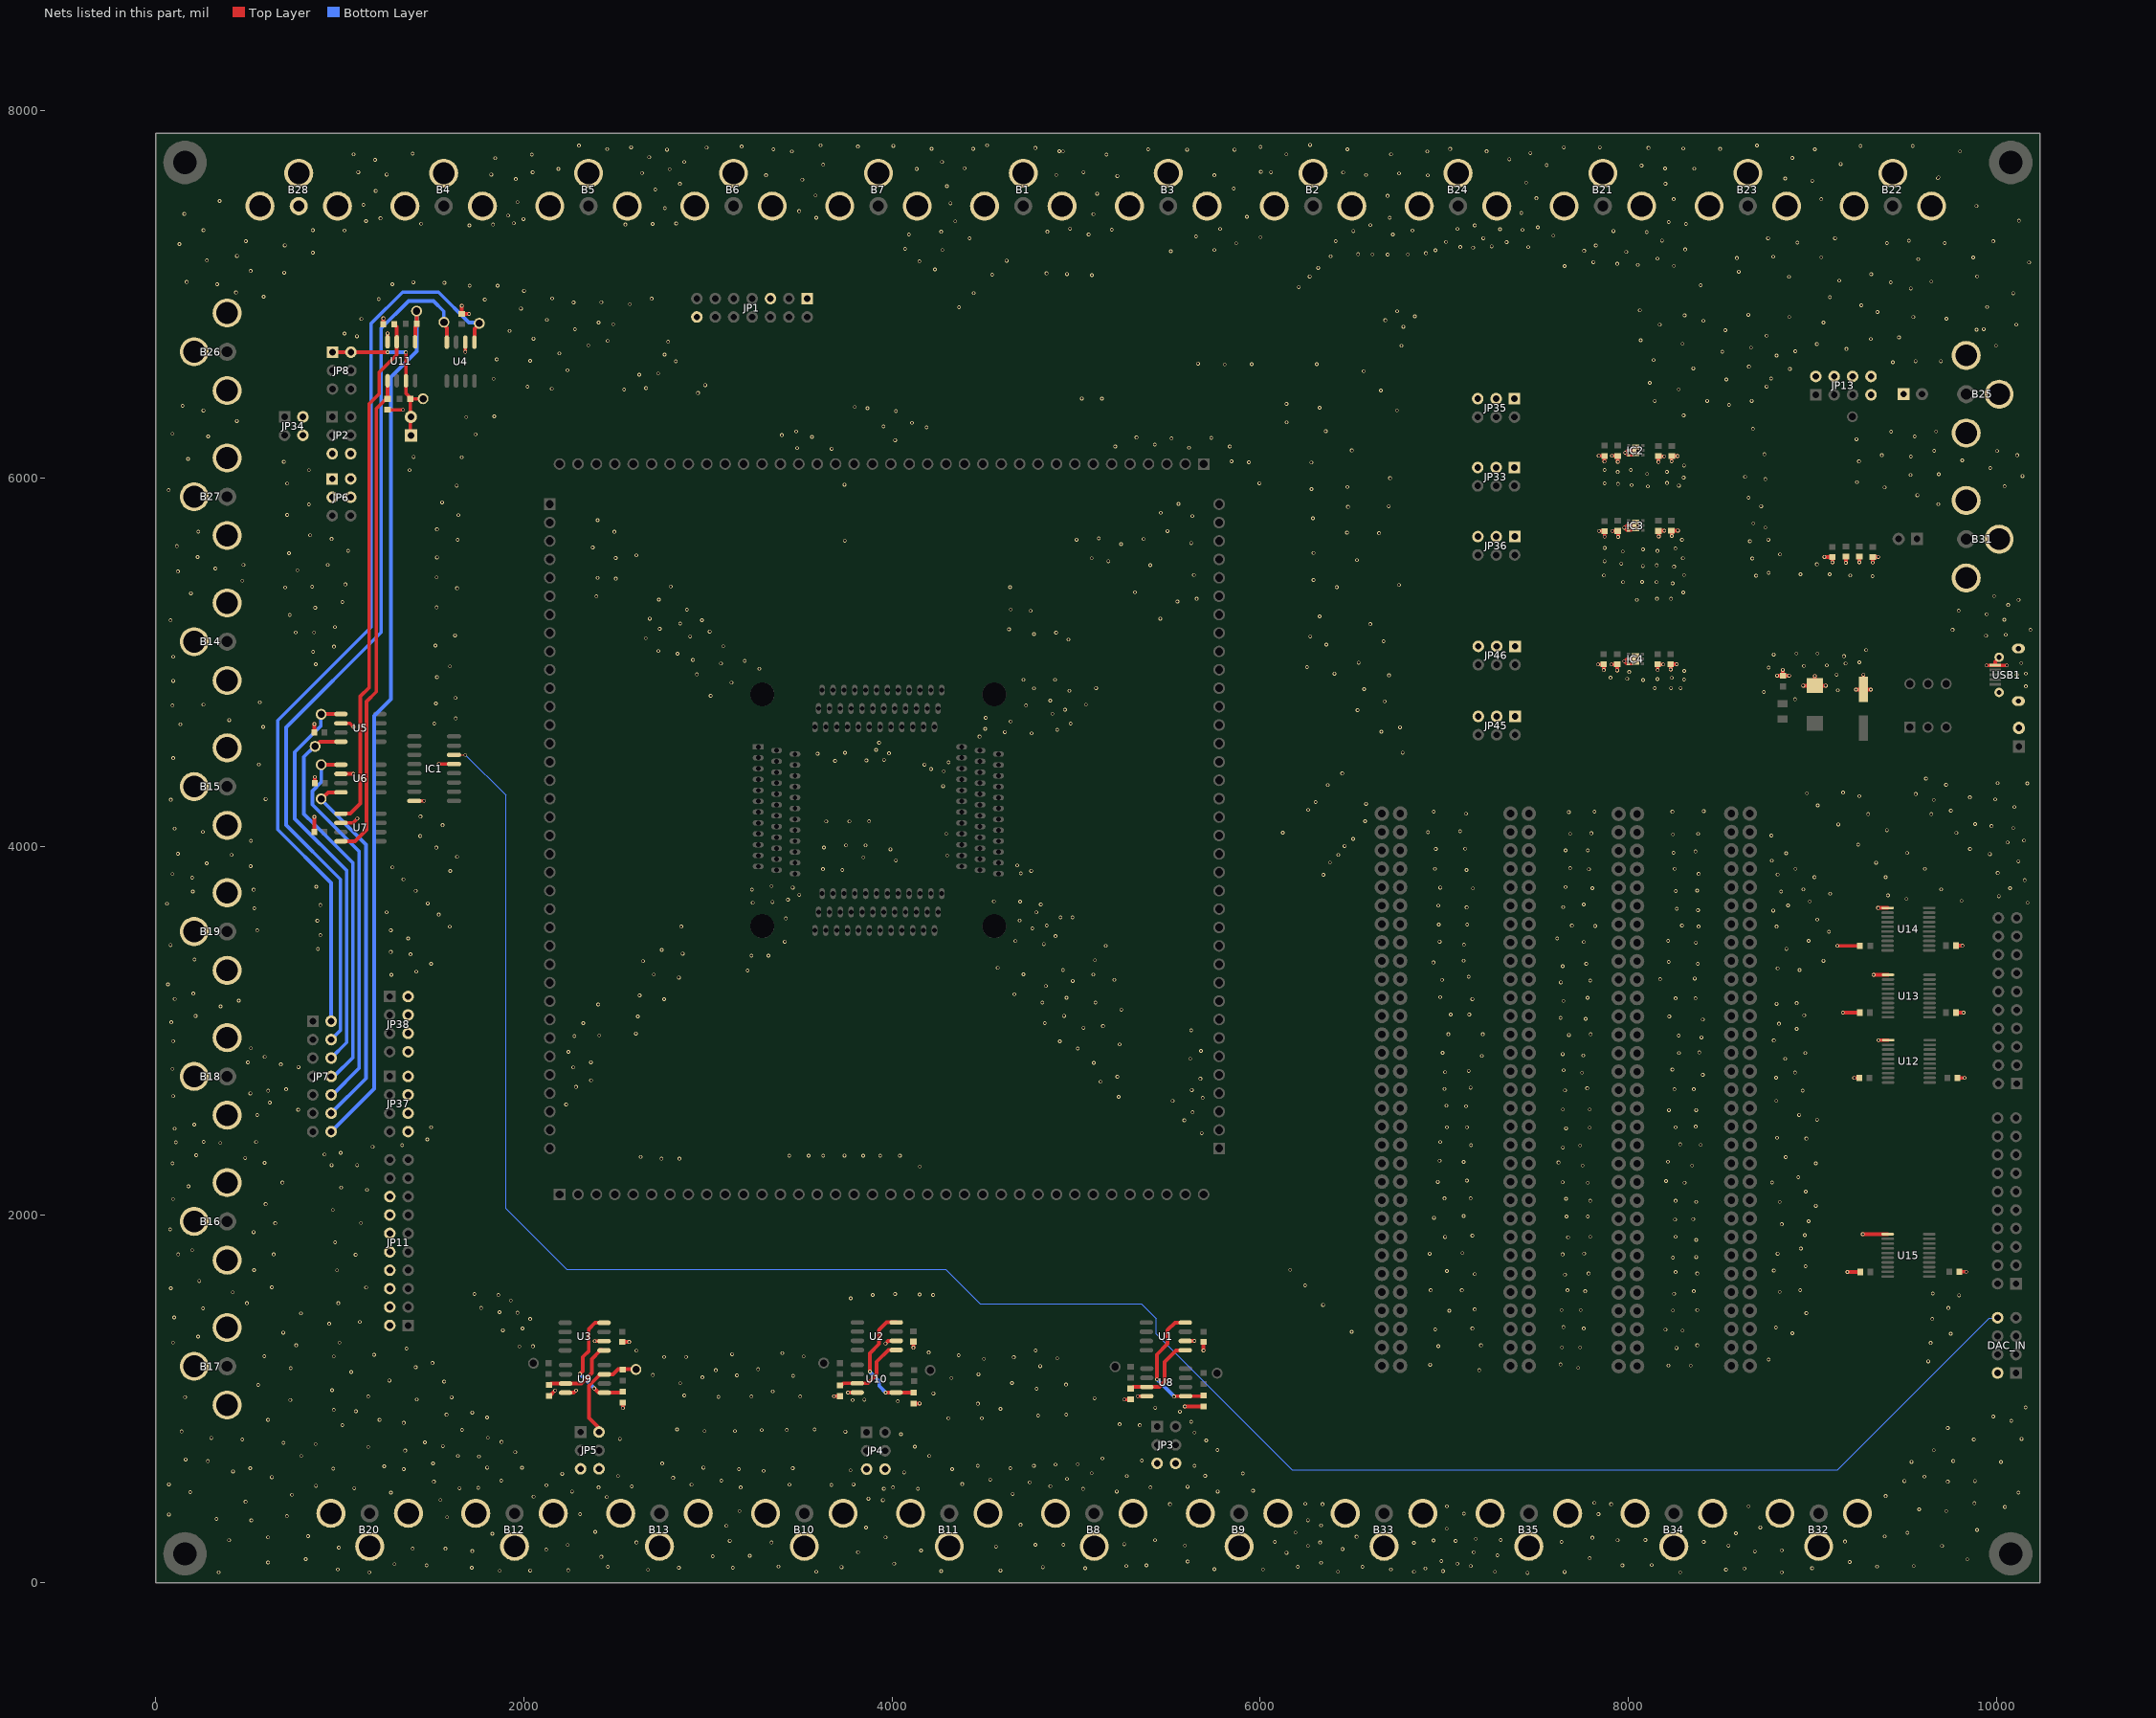
[diagram p0: the nets of this part, all layers, seen from the top]
# Altium PCB MISC62794.PcbDoc (part 3 of 7)
Units mil, origin at the board's own origin, x right, y up, seen from the top; angles counter-clockwise.
Board outline 10236.22 x 7874.02 mil, 4 copper layers (Top Layer, GND, POWER, Bottom Layer); 158 components, 185 nets, 1211 pads, 1759 vias.

## Via types
v1: diameter 20, hole 12, Top Layer to Bottom Layer, 1759 vias

## Nets (pads, with @x,y where several pads share a name; then routed paths per layer and width w, separated by ;. In a path a pad name is that pad's centre, name@x,y a point inside that pad or via, vN(x,y) a via of type N, cw(c..) or ccw(c..) an arc to the next point about the centre after c; other vN are vias at no path point) (continued)
DAC6: JP5.2 R11.1 TP6.1 U9.7 | length 549.3
  Top Layer w20: JP5.2@2407.19,819.02 2407.19,840.81 2353,895 2353,1071 2414,1132 U9.7@2429,1132 ; U9.7@2436.73,1132.67 2483.67,1132.67 2511,1160 TP6.1@2599,1160
DAC7: JP7.2 TP7.1 U4.5 | length 4943.5
  Top Layer w20: U4.5@1730.71,6740.23 1730.71,6812.71 TP7.1@1751,6833
  Bottom Layer w20: JP7.2@952,3051 952,3802 662,4092 662,4685 1169,5192 1169,6841 1340,7012 1535,7012 1700,6847 TP7.1@1752,6847
DAC8: JP7.4 TP8.1 U4.8 | length 4799.4
  Top Layer w20: TP8.1@1566,6833 1580.71,6818.29 U4.8@1580.71,6740.23
  Bottom Layer w20: JP7.4@952,2951 1002,3001 1002,3822 707,4117 707,4647 1223,5163 1223,6177 ; 1223,6188 1223,6177 ; TP8.1@1564,6865 1564,6908 1508,6964 1372,6964 1223,6815 1223,6177
DAC9: JP7.6 TP9.1 U5.5 | length 2171.8
  Top Layer w20: TP9.1@906.54,4719.46 U5.5@1004.93,4719.46
  Bottom Layer w20: TP9.1@896,4714 896,4655 754,4513 754,4151 1036,3869 1036,2935 JP7.6@952,2851
DAC10: JP7.8 TP10.1 U5.8 | length 2132.1
  Top Layer w20: TP10.1@866,4545 890.46,4569.46 U5.8@1004.93,4569.46
  Bottom Layer w20: TP10.1@860,4543 804,4487 804,4177 860,4121 1070,3911 1070,2854 967,2751 JP7.8@952,2751
DAC11: JP7.10 TP11.1 U6.5 | length 2057.5
  Top Layer w20: TP11.1@917.54,4444.46 U6.5@1004.93,4444.46
  Bottom Layer w20: TP11.1@898,4429 898,4350 850,4302 850,4227 1104,3973 1104,2796 959,2651 JP7.10@952,2651
DAC12: JP7.12 TP12.1 U6.8 | length 1981.8
  Top Layer w20: TP12.1@908,4267 935.46,4294.46 U6.8@1004.93,4294.46
  Bottom Layer w20: TP12.1@904,4248 1141,4011 1141,2740 JP7.12@952,2551
DAC13: JP7.14 R13.2 TP13.1 U11.1 | length 4828.2
  Top Layer w20: U11.1@1408.29,6741.99 1408.29,6820.29 1417,6829 TP13.1@1417,6914
  Bottom Layer w20: JP7.14@952,2451 1185,2684 1185,4710 1276,4801 1276,6550 1417,6691 TP13.1@1417,6911
DAC14: JP8.1 JP8.2 JP20.1 JP20.2 R15.1 TP14.1 U11.7 | length 923.6
  Top Layer w20: JP8.1@959,6686.02 1006,6686.02 JP8.2@1059,6686.02 ; JP8.2@1066.98,6686.02 JP8.2@1059,6686.02 ; v1(1257.98,6686.02) JP8.2@1059,6686.02 ; v1@1358.29,6683.29 U11.7@1358.29,6530.77 1358.29,6461.71 R15.1@1386,6434 ; JP20.1@1381.95,6241.95 R15.1@1381.95,6432.38 TP14.1@1448.38,6432.38
  Bottom Layer w20: v1(1257.98,6686.02) v1@1357,6686.02
  other v1: 1358,6685
DAC_OUT1: R2.1 U1.5 U8.3 | length 432.4
  Top Layer w20: R2.1@5303,1055 5311.67,1063.67 U8.3@5383.51,1063.67 5451.67,1063.67 5481,1093 5481,1200 5543,1262 U1.5@5587,1262
DAC_OUT2: R4.1 U1.8 U8.5 | length 691.7
  Top Layer w20: v1(5439,1105) 5439,1240 5497,1298 5497,1373 5537.67,1413.67 U1.8@5592.73,1413.67 ; v1(5532,1012) v1@5533,1012 ; v1@5533,1013 5533.67,1013.67 U8.5@5594.73,1013.67 R4.1@5687.33,1013.67
  Bottom Layer w20: v1(5439,1105) v1(5532,1012)
DAC_OUT3: R6.1 U2.5 U10.3 | length 399.7
  Top Layer w20: R6.1@3729,1078 3734.67,1083.67 U10.3@3810.51,1083.67 U10.3@3823,1083.67 ; U10.3@3823,1084 3868,1084 3916,1132 3916,1201 3980,1265 U2.5@4011,1265
DAC_OUT4: R8.1 U2.8 U10.5 | length 655.7
  Top Layer w20: v1(3879,1148) 3879,1247 3929,1297 3929,1373 3970.67,1414.67 U2.8@4022.73,1414.67 ; v1(3965.33,1033.67) U10.5@4021.73,1033.67 R8.1@4116.67,1033.67
  Bottom Layer w20: v1@3880,1146 3930,1096 3930,1069 v1(3965.33,1033.67)
DAC_OUT5: R10.1 U3.5 U9.3 | length 403.6
  Top Layer w20: R10.1@2140,1075 2147.67,1082.67 U9.3@2225.51,1082.67 2310.67,1082.67 2368,1140 2368,1216 U3.5@2413,1261 ; U3.5@2413,1264 U3.5@2422,1264
DAC_OUT6: R12.1 U3.8 U9.5 | length 633.7
  Top Layer w20: v1@2302,1134 v1@2302.5,1134.5 ; v1(2303,1134) v1@2302.5,1134.5 ; v1(2381,1056) 2404.33,1032.67 U9.5@2436.73,1032.67 R12.1@2531.67,1032.67 ; U3.8@2434.73,1412.67 2385.67,1412.67 2352,1379 2352,1260 2319,1227 2319,1151 v1@2302.5,1134.5
  Bottom Layer w20: v1(2303,1134) v1(2381,1056)
DAC_OUT13: R14.1 U7.5 U11.3 | length 2816.8
  Top Layer w20: U7.5@1004.93,4178.46 1055.46,4178.46 1111,4234 1111,4816 1158,4863 1158,6404 1213,6459 1213,6577 1307,6671 1307,6825 R14.1@1296,6836
DAC_OUT14: R16.1 U7.8 U11.5 | length 2649.2
  Top Layer w20: U7.8@1004.93,4028.46 1082.46,4028.46 1144,4090 1144,4788 1197,4841 1197,6378 1259,6440 U11.5@1259,6527
DCDC_OUT: JP13.7 JP30.1
DIO: DAC_IN.8 IC1.14 | length 11690.6
  Top Layer w6: IC1.14@1619.33,4498.08 v1(1681.08,4498.08)
  Bottom Layer w6: v1(1681.08,4498.08) 1901,4278.16 1901,2033 2232,1702 4292,1702 4478.5,1515.5 5353.5,1515.5 5434,1435 5434,1353 6173,614 9138,614 9961,1437 DAC_IN.8@9997,1437
GND: B1.2 B1.3 B1.4 B2.2 B2.3 B2.4 B3.2 B3.3 B3.4 B4.2 B4.3 B4.4 B5.2 B5.3 B5.4 B6.2 B6.3 B6.4 B7.2 B7.3 B7.4 B8.2 B8.3 B8.4 B9.2 B9.3 B9.4 B10.2 B10.3 B10.4 B11.2 B11.3 B11.4 B12.2 B12.3 B12.4 B13.2 B13.3 B13.4 B14.2 B14.3 B14.4 B15.2 B15.3 B15.4 B16.2 B16.3 B16.4 B17.2 B17.3 B17.4 B18.2 B18.3 B18.4 B19.2 B19.3 B19.4 B20.2 B20.3 B20.4 B21.2 B21.3 B21.4 B22.2 B22.3 B22.4 B23.2 B23.3 B23.4 B24.2 B24.3 B24.4 B25.2 B25.3 B25.4 B26.2 B26.3 B26.4 B27.2 B27.3 B27.4 B28.1 B28.2 B28.3 B28.4 B31.2 B31.3 B31.4 B32.2 B32.3 B32.4 B33.2 B33.3 B33.4 B34.2 B34.3 B34.4 B35.2 B35.3 B35.4 C1.1 C2.1 C3.1 C4.1 C5.1 C6.1 C7.1 C8.2 C9.2 C10.2 C11.2 C20.2 C21.2 C22.2 C23.2 C24.2 C25.2 C26.2 C27.2 C28.2 C30.1 C31.2 C32.1 C33.2 C34.1 C35.2 C36.1 C37.2 C38.2 C39.2 C40.2 C41.2 D1.2 DAC_IN.2 IC1.8 IC1.13 IC2.2 IC2.3 IC2.7 IC3.2 IC3.3 IC3.7 IC4.2 IC4.3 IC4.7 JP1.1 JP1.5 JP1.14 JP2.5 JP2.6 JP3.5 JP3.6 JP4.5 JP4.6 JP5.5 JP5.6 JP6.1 JP6.2 JP6.3 JP6.4 JP11.2 JP11.4 JP11.6 JP11.8 JP11.10 JP11.12 JP11.14 JP11.16 JP13.2 JP13.4 JP13.6 JP13.8 JP32.2 JP33.1 JP33.3 JP33.5 JP34.2 JP34.4 JP35.1 JP35.3 JP35.5 JP36.1 JP36.3 JP36.5 JP37.2 JP37.4 JP37.6 JP37.8 JP38.2 JP38.4 JP38.6 JP38.8 JP45.1 JP45.3 JP45.5 JP46.1 JP46.3 JP46.5 R2.2 R4.2 R6.2 R8.2 R10.2 R12.2 R14.2 R16.2 R20.2 U1.6 U2.6 U3.6 U4.6 U5.6 U6.6 U7.6 U8.4 U9.4 U10.4 U11.4 U12.11 U13.11 U14.11 U15.11 USB1.5 USB1.6 USB1.7 USB1.8 USB1.9 | length 4162.4
  Top Layer w16: v1@7978,5006 7990.58,4993.42 IC4.3@8000.61,4993.42 IC4.7@8019.58,4993.42 ; v1(7978,5007) 7990.02,5019.02 IC4.2@8000.61,5019.02 IC4.7@8021.98,5019.02 ; v1@7978,5731 7990.58,5718.42 IC3.3@8000.61,5718.42 ; v1(7978,5732) 7990.02,5744.02 IC3.2@8000.61,5744.02 ; v1@7983,6139 7995.58,6126.42 IC2.3@8005.61,6126.42 ; v1(7983,6140) 7995.02,6152.02 IC2.2@8005.61,6152.02 ; IC3.3@8001.61,5718.42 8018.42,5718.42 IC3.7@8022,5722 ; IC3.2@8001.61,5744.02 IC3.7@8023.98,5744.02 ; IC2.3@8002.61,6126.42 IC2.7@8023.42,6126.42 ; IC2.2@8002.61,6152.02 IC2.7@8023.02,6152.02
  Top Layer w20: C7.1@860.98,4079.46 v1(860.98,4160.98) ; C5.1@860.98,4619.46 v1(860.98,4664.98) ; C6.1@862.98,4344.46 v1(862.98,4377.98) ; U7.6@1004.93,4128.46 1070.46,4128.46 v1(1094,4152) ; U6.6@1004.93,4394.46 v1(1072.54,4394.46) ; U5.6@1004.93,4669.46 1054.54,4669.46 v1(1074,4650) ; R14.2@1235.63,6838.38 v1(1235.63,6869.63) ; R16.2@1258.29,6372.72 1259.01,6372 v1(1343,6372) ; U11.4@1258.29,6741.99 v1(1258.29,6787.71) ; IC1.8@1403.94,4248.08 v1(1456.92,4248.08) ; v1(1537.08,4448.08) IC1.13@1619.33,4448.08 ; v1(1662,6938) C4.1@1662,6893.56 v1(1701.44,6893.56) ; v1(1680.71,6687.29) U4.6@1680.71,6740.23 ; R10.2@2135.12,1015.01 2139.01,1015.01 v1(2169,1045) ; U9.4@2225.51,1032.67 2270.67,1032.67 v1(2283,1045) ; v1(2384.33,1312.67) U3.6@2434.73,1312.67 ; C3.1@2534.12,1308.11 v1(2570.89,1308.11) ; v1(2537,949) R12.2@2537,978.34 ; v1(3684.01,1014.01) R6.2@3717.12,1014.01 ; v1(3760.33,1033.67) U10.4@3810.51,1033.67 ; v1(3964,1300) 3978.67,1314.67 U2.6@4022.73,1314.67 ; v1(4116.12,1277.12) C2.1@4116.12,1310.11 ; R8.2@4118,974.34 v1(4149.34,974.34) ; v1(5260.99,996.01) R2.2@5296.12,996.01 ; v1(5334,1014) 5334.33,1013.67 U8.4@5383.51,1013.67 ; v1(5590.66,958.34) R4.2@5693,958.34 ; U1.6@5592.73,1313.67 v1(5643.33,1313.67) ; v1(5692.12,1262.12) C1.1@5692.12,1309.11 ; v1(7835.54,4989.46) C41.2@7866.56,4989.46 v1(7866.56,4958.44) ; v1(7839.54,6122.46) 7870.56,6122.46 v1(7870.56,6091.44) ; v1(7840.54,5714.46) 7871.56,5714.46 v1(7871.56,5683.44) ; v1(7907.54,4989.46) C40.2@7939.56,4989.46 v1(7939.56,4957.44) ; v1(7911.54,6122.46) 7943.56,6122.46 v1(7943.56,6090.44) ; v1(7912.54,5714.46) 7944.56,5714.46 v1(7944.56,5682.44) ; v1(8159.56,4958.44) C38.2@8159.56,4989.46 v1(8190.54,4989.46) ; v1(8164.56,6089.44) C24.2@8164.56,6120.46 v1(8195.54,6120.46) ; v1(8165.56,5684.44) 8165.56,5715.46 v1(8196.54,5715.46) ; v1(8230.56,4961.56) C39.2@8230.56,4990.46 v1(8263.54,4990.46) ; v1(8235.56,6092.56) 8235.56,6121.46 v1(8268.54,6121.46) ; v1(8236.56,5687.56) 8236.56,5716.46 v1(8269.54,5716.46) ; v1(8808.34,4928.66) R20.2@8840,4928.66 ; v1(8840,4960) R20.2@8840,4928.66 ; v1(8874.34,4928.66) R20.2@8840,4928.66 ; v1(8950.98,4874.02) D1.2@9014,4874.02 ; v1(9014,4927) D1.2@9014,4874.02 ; v1(9065.59,5573.41) C10.2@9109.29,5573.41 v1(9109.29,5544.29) ; v1(9072.98,4874.02) D1.2@9014,4874.02 ; v1(9135.99,3460.01) C34.1@9259.44,3460.01 ; v1(9165.99,3098.01) C32.1@9257.44,3098.01 ; v1(9182.29,5541.29) C9.2@9182.29,5574.41 ; v1(9191.01,1689.01) C36.1@9260.44,1689.01 ; v1(9228,2743) C30.1@9255.44,2743.01 ; v1(9237.12,4853.12) C20.2@9278,4853.12 ; v1(9255.29,5544.29) C8.2@9255.29,5575.41 ; v1(9274.83,1894.17) U15.11@9409.97,1894.17 ; v1(9278,4934) C20.2@9278,4853.12 ; v1(9317.88,4853.12) C20.2@9278,4853.12 ; v1(9328.29,5542.71) C11.2@9328.29,5573.41 v1(9358.59,5573.41) ; v1(9333.17,3303.17) U13.11@9410.97,3303.17 ; v1(9357.83,3666.17) U14.11@9408.97,3666.17 ; v1(9359.83,2948.17) U12.11@9411.97,2948.17 ; C33.2@9780.56,3098.01 v1(9821.99,3098.01) ; C35.2@9780.56,3461.01 v1(9815.99,3461.01) ; C31.2@9789.56,2743.01 v1(9827.99,2743.01) ; C37.2@9799.56,1690.01 v1(9837.01,1690.01) ; v1(9946.06,4984.06) USB1.5@9994.63,4984.06 ; USB1.6@10005,5015 9994.63,5004.63 USB1.5@9994.63,4984.06 ; v1(10057.94,4984.06) USB1.5@9994.63,4984.06
  other v1: 7453,54 341,57 1159,57 8282,57 8834,57 7654,59 3588,60 6423,60 6836,60 7276,60 4266,64 6993,64 1868,65 2034,67 4589,67 2240,68 2674,70 8531,71 988,73 6015,73 6710,73 5751,74 6898,78 8631,78 5049,79 8999,79 1716,82 2841,82 3134,82 3725,85 4819,85 2456,87 6205,87 6556,87 3383,88 9352,88 5273,91 7144,91 9551,91 1470,95 5382,95 7968,95 8127,96 1296,101 4011,104 7071,104 6331,109 609,110 9203,113 5606,116 6985,118 9842,127 814,129 7791,133 2420,141 3025,144 3227,147 7289,149 6143,163 3815,166 7161,166 8688,171 1719,172 4157,175 8834,177 2120,180 6447,183 1395,185 1573,185 994,191 4564,197 6259,200 9705,200 8545,202 5591,203 2237,205 4779,207 4931,207 5261,210 6835,217 2611,219 3345,219 6326,219 6080,222 7637,222 8410,222 9178,224 7062,227 3118,228 6942,230 397,231 5429,231 7942,231 7307,233 8093,233 7172,239 7805,245 609,247 3964,247 6524,250 9394,252 826,253 1828,266 8585,269 9517,272 6192,273 2387,277 9895,287 7013,294 3858,300 8718,301 3100,309 6331,312 4698,315 518,339 6259,340 329,347 1582,356 711,362 70,371 2305,373 7838,373 7107,376 3171,390 9728,390 9581,399 10047,412 7015,416 8654,416 5510,427 6339,427 7907,427 6245,429 9881,432 7816,434 487,440 3950,449 1546,450 3871,457 2450,465 2052,468 9399,471 739,478 4655,483 1277,490 10120,490 186,493 2261,496 5221,496 5769,496 5961,500 5037,510 3955,511 4140,511 1078,514 1650,514 1751,516 2405,518 3177,518 4005,518 5404,518 5605,522 2586,524 4860,525 870,527 2122,530 3670,532 2910,533 3442,533 70,535 3790,535 4381,536 4748,546 1510,549 9736,549 9501,553 9884,553 1876,555 3072,555 4533,561 4950,564 2810,570 630,574 9609,577 2510,580 5275,580 5701,581 2207,592 5906,594 5084,595 4065,600 419,605 3302,608 3774,611 1346,617 3168,617 4326,617 963,620 512,623 3460,623 4642,623 1989,625 1800,626 2975,626 1240,633 4465,636 4770,636 5643,636 4888,642 5009,645 2751,648 1505,649 10025,656 9539,657 282,661 9766,662 5357,664 161,670 5143,676 1755,686 789,689 1641,689 4202,689 1952,710 1354,718 9660,720 5768,721 1153,738 4123,740 1559,743 867,754 693,760 1461,763 1878,765 5707,773 469,779 9878,779 2521,782 10137,782 300,787 1803,788 4048,807 5643,816 3746,821 139,822 2981,824 3146,824 3292,829 3428,830 1663,831 2831,833 3579,833 9736,841 5346,856 1013,857 5236,861 1346,869 5625,875 10081,880 609,885 1215,885 4306,894 4487,894 1799,898 9983,903 4793,909 1579,913 4946,914 1719,925 5564,930 1086,932 966,939 4589,945 5430,951 10159,953 4466,973 4031,986 730,993 3786,993 3849,995 1417,996 5100,1003 1606,1008 158,1009 3056,1010 1153,1012 3236,1012 3501,1012 2871,1018 4224,1029 3351,1040 957,1046 4785,1054 555,1075 4945,1077 2848,1084 4651,1085 1566,1093 1268,1099 4322,1113 2969,1116 3462,1124 3157,1127 2700,1129 4469,1133 1061,1145 3042,1155 7190,1155 3272,1160 732,1166 7728,1167 1411,1171 4805,1177 8218,1180 8339,1180 6924,1185 7632,1186 1502,1194 9630,1203 8763,1213 4499,1217 4897,1219 4661,1225 2761,1227 2880,1227 966,1230 3519,1230 589,1231 4361,1236 1185,1239 3131,1242 3403,1248 4199,1251 2611,1261 4780,1262 1361,1273 8262,1276 7640,1279 7739,1279 1975,1284 2048,1285 6968,1286 762,1290 7200,1290 8375,1290 9643,1303 92,1305 997,1305 229,1338 9752,1353 8892,1356 692,1359 6497,1364 8295,1370 1885,1372 8202,1375 6951,1377 7153,1381 7758,1381 1992,1382 8802,1387 7648,1389 941,1407 1108,1417 2033,1433 9652,1433 99,1442 788,1464 8968,1465 1964,1467 1867,1470 7028,1478 8243,1479 7637,1482 7741,1482 8375,1482 7166,1485 256,1491 1767,1493 9739,1493 6342,1510 494,1519 991,1519 1928,1534 3775,1546 9798,1562 1860,1563 3895,1564 4223,1564 4149,1566 1730,1569 4016,1569 8249,1570 9655,1572 417,1578 8823,1581 7766,1584 8356,1584 6927,1589 7096,1589 7670,1589 8935,1590 81,1600 1142,1604 630,1605 6244,1616 235,1640 7656,1674 7166,1677 7785,1680 8375,1680 8257,1688 7015,1694 8791,1696 984,1698 533,1699 6163,1700 8963,1720 8243,1767 8369,1770 1085,1782 121,1784 640,1784 7643,1784 6921,1788 8812,1788 7760,1789 7099,1791 196,1807 8938,1816 974,1850 8369,1863 7673,1877 7005,1879 7793,1880 8257,1880 7153,1886 8959,1889 530,1905 77,1920 8834,1948 648,1953 1114,1955 8980,1964 8254,1973 8353,1976 6944,1983 7665,1990 7780,1990 7106,1993 961,2025 9019,2048 596,2057 8369,2069 8823,2069 7793,2075 8257,2075 92,2085 7662,2086 7002,2088 7143,2088 8965,2125 1147,2134 1006,2147 176,2154 7780,2173 8306,2173 687,2174 8781,2175 7643,2176 6965,2178 8205,2182 7123,2185 8924,2203 4151,2262 7752,2267 8347,2267 954,2269 1093,2269 90,2279 9019,2279 590,2281 7621,2283 7106,2286 8216,2288 6975,2293 2747,2304 2844,2304 485,2308 8856,2312 2634,2314 3441,2320 3546,2320 3626,2320 3843,2320 3935,2320 4042,2320 3741,2321 219,2323 916,2327 1004,2336 7645,2365 1177,2368 7739,2376 1338,2377 7146,2377 8394,2379 8282,2382 350,2389 108,2393 544,2394 6978,2394 259,2396 1474,2409 8968,2413 8809,2418 5682,2443 101,2467 7662,2469 7791,2472 1495,2475 7015,2475 7123,2475 8257,2475 8367,2478 208,2489 5588,2513 9026,2516 550,2541 8929,2542 5633,2556 8221,2568 8369,2568 773,2570 7645,2571 7791,2571 7119,2589 7012,2592 2229,2598 618,2609 5524,2618 8805,2618 5687,2634 5231,2640 93,2644 513,2659 610,2673 8948,2674 7656,2675 5628,2677 707,2681 8251,2681 8356,2681 7002,2683 7777,2686 7143,2690 2282,2694 5133,2722 2364,2730 5675,2738 8803,2744 5224,2749 8405,2760 7749,2771 8906,2772 7005,2774 7133,2781 7649,2784 8240,2788 90,2792 2268,2800 774,2802 679,2816 5096,2825 500,2827 2363,2828 5620,2847 8853,2847 591,2857 7204,2862 7756,2865 7644,2872 8276,2878 8962,2878 6991,2879 8386,2881 2241,2884 5678,2890 5009,2903 516,2904 5236,2925 4911,2942 93,2943 8791,2946 8398,2963 2274,2970 8274,2973 2409,2974 7678,2976 7022,2980 7210,2980 7796,2980 2608,2984 5625,3001 8915,3009 5040,3015 5146,3024 8819,3037 2322,3040 4829,3040 83,3045 8405,3060 7769,3064 7632,3069 2618,3077 8223,3077 215,3079 4934,3080 8956,3083 7035,3087 7136,3087 5245,3114 351,3131 2403,3142 8806,3145 8915,3149 4816,3152 5105,3152 7648,3161 450,3163 2761,3170 7153,3171 102,3172 8257,3175 8365,3175 4948,3178 7779,3178 6978,3182 2628,3191 4664,3198 203,3201 4835,3242 65,3251 7634,3262 4981,3270 7793,3272 5208,3276 6988,3276 8173,3279 8361,3283 2841,3288 7133,3293 1279,3303 2705,3304 5093,3304 4714,3306 1414,3320 3215,3326 4928,3329 8931,3329 8812,3338 4574,3341 7644,3350 1495,3363 7772,3363 8378,3363 6941,3370 8220,3373 2646,3377 9061,3379 7106,3380 5102,3382 209,3386 3236,3407 3328,3407 1383,3414 2862,3418 1276,3427 2748,3438 880,3443 8859,3444 5161,3460 79,3465 7107,3466 4824,3470 8368,3478 7759,3481 3417,3483 6975,3483 4670,3486 8217,3488 8980,3488 1370,3501 7614,3501 4888,3513 893,3518 9091,3537 550,3544 1276,3545 4762,3555 1596,3564 2854,3565 8382,3565 8806,3565 7820,3568 7694,3570 4840,3571 8292,3571 6970,3576 7125,3576 877,3597 4693,3598 9027,3603 3423,3609 4915,3615 4980,3615 1537,3630 1253,3642 4783,3642 8788,3652 8379,3654 8264,3662 534,3664 7122,3669 7646,3671 6968,3679 8868,3680 893,3682 4808,3685 7758,3685 60,3689 1477,3691 3243,3694 10170,3694 3350,3699 4695,3701 4553,3702 8987,3702 9811,3705 3434,3711 9512,3715 10014,3730 9411,3735 3496,3738 9097,3744 200,3755 8831,3755 8259,3758 1411,3759 8374,3761 531,3765 3238,3766 8952,3767 9700,3767 7156,3772 7805,3774 10075,3774 3460,3777 6979,3777 7659,3780 871,3781 3345,3785 10154,3817 1345,3822 196,3831 9012,3833 9399,3833 6343,3846 8812,3848 90,3850 8383,3851 4699,3854 10008,3856 1599,3867 4756,3868 3730,3872 7121,3872 7786,3876 3624,3877 6950,3879 8253,3879 8909,3879 9612,3879 7684,3882 1285,3887 514,3893 4680,3897 276,3909 9347,3912 6379,3913 10120,3920 8780,3923 4021,3925 3844,3941 1636,3944 4299,3952 410,3954 6424,3954 9965,3959 119,3961 8858,3963 9515,3965 8246,3966 8365,3973 7659,3979 7780,3979 3991,3985 6954,3987 9857,3987 7114,3988 1523,3994 3630,3995 6459,4003 3750,4006 3856,4006 9249,4010 10061,4022 516,4031 10151,4032 6505,4041 1436,4057 8778,4060 8243,4066 4294,4069 7684,4069 8380,4069 7799,4072 9783,4074 6123,4075 6912,4078 255,4079 7086,4083 9405,4089 101,4097 10092,4100 9974,4111 1557,4116 9141,4120 9885,4122 3642,4136 3768,4136 3875,4137 6570,4138 1437,4163 9304,4176 9647,4176 7118,4178 7677,4187 8240,4189 6943,4190 7817,4190 8410,4192 9753,4195 6261,4199 10098,4214 9030,4223 6575,4232 6301,4242 9660,4253 81,4254 9994,4256 596,4258 9856,4267 9256,4274 9562,4285 8971,4290 9167,4293 4277,4328 6367,4334 9727,4335 10168,4343 10007,4344 9618,4369 6446,4397 4281,4409 4211,4421 4176,4445 559,4446 4307,4457 3690,4465 3860,4468 3956,4471 94,4480 3595,4504 3983,4506 3744,4509 6774,4510 3913,4525 3929,4564 4475,4597 4758,4615 4613,4622 6658,4624 4897,4634 4506,4639 6760,4648 582,4650 133,4664 1512,4668 4970,4668 4644,4680 398,4687 1629,4696 4509,4699 4871,4721 6529,4741 4939,4743 90,4766 4728,4766 258,4771 5053,4771 1521,4777 564,4784 6676,4789 4859,4793 8906,4800 1627,4807 3014,4819 8737,4840 4963,4846 9139,4849 6565,4855 4771,4859 8144,4860 5108,4861 8233,4861 8285,4861 10161,4870 3127,4890 94,4900 8081,4905 4714,4906 4885,4906 8303,4907 8159,4910 7994,4911 8236,4916 7904,4917 1527,4920 6700,4930 10111,4933 9132,4934 2939,4935 6404,4939 10161,4940 8005,4948 8304,4954 3279,4966 8763,4972 6254,4975 1598,4979 8955,4981 9079,4984 868,4990 3070,4994 9181,4994 10136,4997 6535,4999 8031,4999 9256,5001 3199,5009 2918,5014 8048,5018 94,5031 9172,5034 8031,5038 8790,5043 2834,5048 8914,5049 9028,5049 854,5058 2730,5062 9293,5067 967,5086 3082,5088 1518,5092 6359,5097 6670,5115 4958,5124 2661,5132 2903,5142 6272,5142 9944,5145 1625,5147 10051,5150 4771,5154 4891,5162 759,5163 859,5163 3009,5168 9762,5177 10185,5177 4635,5180 2737,5183 972,5192 6598,5208 2848,5211 79,5229 2967,5230 10044,5232 2683,5238 5457,5238 6323,5250 727,5258 9948,5262 4752,5280 9795,5281 2885,5287 4645,5288 865,5297 1525,5299 10064,5312 1013,5328 5550,5331 8047,5340 10121,5340 2733,5341 5655,5346 8156,5346 8233,5346 2393,5359 9988,5361 190,5376 8299,5380 5319,5382 1636,5403 702,5408 4641,5409 6416,5409 849,5412 2797,5413 6754,5421 1029,5424 8241,5430 7972,5436 8154,5436 8075,5438 469,5444 6290,5448 2499,5455 2400,5460 1525,5462 9327,5469 8695,5471 7868,5473 9206,5473 5640,5475 8303,5475 8936,5479 9095,5479 8763,5487 119,5494 768,5501 323,5510 8249,5520 8079,5524 8155,5528 5403,5529 475,5530 933,5530 9025,5533 7962,5537 5175,5550 7871,5550 6526,5556 8674,5565 5084,5566 8297,5566 2498,5568 1527,5571 226,5573 2610,5582 8825,5587 723,5594 6290,5595 7970,5603 8159,5606 1044,5607 8080,5614 8256,5619 7872,5622 2373,5625 113,5632 5244,5643 5625,5649 8661,5659 3743,5662 1639,5666 8292,5666 5002,5667 8761,5667 5367,5670 954,5671 5123,5674 838,5691 6646,5702 6472,5705 2491,5710 230,5711 5496,5714 1527,5723 8032,5725 8745,5733 8049,5744 8680,5756 8032,5764 2400,5773 6287,5783 5631,5795 1643,5800 713,5802 5460,5813 6477,5845 6699,5849 8722,5849 831,5859 9685,5860 5556,5861 1555,5870 8654,5895 9571,5909 69,5936 6279,5942 9393,5951 6474,5954 8107,5956 10045,5957 1634,5961 8275,5961 8018,5964 3741,5966 7944,5970 713,5972 7871,5973 5996,5974 8211,5975 9243,5980 8745,5996 6706,6001 8301,6004 8635,6008 10142,6013 9534,6019 9687,6023 8103,6024 7943,6035 8210,6036 831,6045 1378,6045 7871,6046 8014,6046 9967,6056 8303,6070 6278,6086 5939,6088 695,6090 9254,6092 5844,6093 9815,6098 174,6106 1661,6115 1400,6117 9535,6119 9378,6126 10113,6126 8740,6131 8033,6133 10004,6149 9663,6150 6498,6152 8050,6152 3672,6161 3484,6164 5613,6167 8033,6172 5212,6173 5835,6173 5427,6184 4016,6208 9240,6213 5518,6217 5734,6220 5328,6222 3565,6225 283,6228 9556,6228 3401,6235 1736,6240 90,6242 9429,6254 3479,6255 9673,6255 6356,6257 8677,6269 4187,6277 3953,6283 4108,6302 6144,6305 439,6312 1686,6333 1838,6337 8301,6342 4021,6366 258,6369 6743,6370 3866,6381 6323,6384 3797,6388 144,6394 8547,6400 6143,6405 8144,6421 8429,6421 8671,6421 5140,6433 5031,6434 2945,6464 6656,6478 2544,6483 8274,6484 2151,6487 2663,6491 2019,6498 8752,6499 2984,6507 8117,6519 8533,6537 1834,6541 8776,6543 2626,6563 2729,6570 6563,6583 2236,6588 8878,6595 8354,6598 8656,6607 5807,6619 5954,6621 6307,6621 5662,6624 9438,6631 2825,6636 9561,6637 9699,6637 2033,6639 8138,6643 1852,6647 8806,6667 2764,6673 2192,6679 8511,6688 8908,6691 9186,6703 8667,6710 6768,6721 9998,6721 2349,6723 9025,6730 8295,6731 2783,6742 2455,6747 8068,6751 9318,6757 2051,6759 9471,6766 1092,6772 8752,6775 1024,6787 1921,6801 8527,6805 9893,6808 2276,6810 9932,6811 6778,6824 8171,6835 10109,6835 2484,6838 2405,6847 9061,6847 8408,6856 6680,6859 2124,6861 1116,6866 9729,6868 8875,6877 9549,6877 6840,6881 8306,6886 8653,6889 9354,6904 6744,6908 8063,6913 1983,6923 4364,6930 9950,6931 9267,6940 2575,6947 2269,6956 2420,6957 1787,6972 1210,6974 2693,6976 2153,6978 9096,6985 585,6987 10092,7006 4443,7007 435,7010 2000,7019 9535,7032 6210,7040 1704,7047 1856,7047 8394,7050 332,7055 1284,7055 1567,7063 9426,7065 1398,7066 167,7067 9647,7069 9147,7074 8874,7095 6269,7097 9896,7098 5085,7104 4543,7107 9320,7109 4950,7110 4839,7114 697,7118 8601,7123 514,7127 4233,7135 6315,7144 7654,7154 8248,7155 8052,7160 7940,7166 10178,7173 7811,7175 4148,7179 4622,7183 277,7184 9576,7191 8159,7194 8590,7197 9875,7200 9049,7202 8788,7204 6383,7207 440,7209 6693,7216 6610,7217 6803,7217 6532,7218 6901,7223 852,7226 7989,7230 5514,7234 7760,7236 6952,7239 4273,7241 5751,7241 8309,7244 4070,7247 7157,7254 7457,7256 7087,7257 7258,7261 7824,7265 700,7266 127,7273 5869,7277 9405,7278 9720,7278 8919,7281 7339,7284 7010,7285 9983,7288 488,7289 6410,7289 9525,7291 8183,7292 4421,7304 7213,7305 8760,7305 9124,7305 6002,7311 5651,7315 7593,7319 4091,7325 5068,7325 6721,7325 8100,7338 4266,7340 4844,7340 6506,7344 7919,7344 1024,7347 6827,7347 258,7349 852,7349 7425,7350 5193,7351 7303,7354 5782,7355 7072,7355 4967,7357 7509,7364 1703,7375 7166,7375 6599,7376 1832,7379 2551,7379 2699,7382 8313,7382 1441,7384 2827,7385 1944,7386 8220,7393 4343,7397 1141,7398 10123,7400 1997,7409 1220,7413 3588,7416 6704,7416 5928,7421 1913,7428 5094,7436 154,7437 7419,7442 3495,7452 2765,7468 9892,7480 1127,7486 4317,7495 1964,7501 346,7507 8247,7517 9049,7517 7501,7522 6692,7535 3584,7537 5114,7547 1194,7562 2713,7570 5856,7575 4298,7588 2847,7600 8202,7601 7445,7607 9000,7617 3512,7623 1955,7626 8853,7629 9682,7631 9686,7636 5224,7643 6911,7646 3315,7647 5751,7647 4892,7649 6575,7649 1254,7651 1822,7651 6755,7657 2641,7659 6451,7662 2047,7663 1099,7664 5040,7664 6059,7664 6004,7666 2791,7680 2187,7681 4133,7681 8359,7683 8200,7684 4393,7685 8072,7700 7557,7702 3626,7704 9154,7708 2870,7719 4271,7719 1190,7731 7354,7734 1843,7740 8891,7741 2680,7745 2042,7759 5165,7759 1074,7761 6142,7761 6711,7761 1395,7765 7468,7768 3455,7776 4928,7776 6908,7776 9803,7776 7230,7777 4909,7778 2777,7786 5603,7786 5861,7786 3355,7788 5391,7788 6474,7788 9014,7788 2452,7789 7032,7790 8499,7790 4214,7791 4440,7791 8299,7792 4778,7795 8110,7795 2992,7797 2582,7799 7650,7799 7845,7799 6002,7801 3182,7803 3814,7803 9262,7806 9546,7806 4006,7807 2298,7808 8699,7809 3611,7810 4516,7810 6271,7812